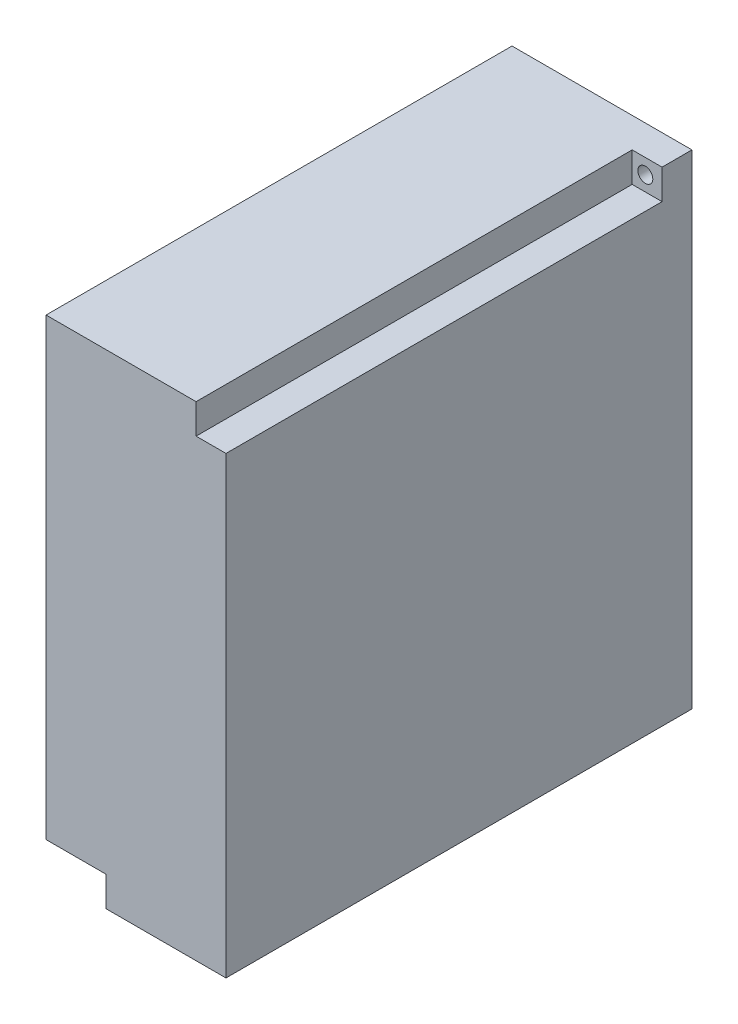
SolidWorks part; units mm, degrees
material "45#"
ref_plane "Front Plane" through (0, 0, 0) normal (0, 0, 1) x (1, 0, 0)
ref_plane "Top Plane" through (0, 0, 0) normal (0, 1, 0) x (1, 0, 0)
ref_plane "Right Plane" through (0, 0, 0) normal (1, 0, 0) x (0, 0, -1)
sketch "Sketch1" plane through (0, 0, 0) normal (0, 0, 1) x (1, 0, 0)
  line L0 (-30.1, 81) -> (30.1, -81) construction
  line L1 (-30.1, 81) -> (30.1, 81)
  line L2 (-30.1, 81) -> (-30.1, -81)
  line L3 (-30.1, -81) -> (30.1, -81)
  line L4 (30.1, 81) -> (30.1, -81)
  dimension "D1" = 60.2
  dimension "D2" = 162
extrude "Extrude1" add sketch "Sketch1" along normal blind 155.9
sketch "Sketch2" plane through (0, 0, 155.9) normal (0, 0, 1) x (1, 0, 0)
  line L1 (-30.1, -81) -> (-10.1, -81)
  line L2 (-30.1, -81) -> (-30.1, -71)
  line L3 (-30.1, -71) -> (-10.1, -71)
  line L4 (-10.1, -81) -> (-10.1, -71)
  line L5 (30.1, 81) -> (20.1, 81)
  line L6 (30.1, 81) -> (30.1, 71)
  line L7 (30.1, 71) -> (20.1, 71)
  line L8 (20.1, 81) -> (20.1, 71)
  dimension "D1" = 10
  dimension "D2" = 10
  dimension "D3" = 20
extrude "Cut-Extrude1" cut sketch "Sketch2" against normal blind 145.9
sketch "Sketch3" plane through (0, 0, 155.9) normal (0, 0, 1) x (1, 0, 0)
  line L0 (-24.5, 76) -> (24.5, -76) construction
  line L1 (-24.5, 76) -> (24.5, 76) construction
  line L2 (-24.5, 76) -> (-24.5, -76) construction
  line L3 (-24.5, -76) -> (24.5, -76) construction
  line L4 (24.5, 76) -> (24.5, -76) construction
  circle A0 centre (24.5, 76) radius 2.5
  circle A1 centre (-24.5, -76) radius 2.5
  dimension "D3" = 5
  dimension "D1" = 49
  dimension "D2" = 152
extrude "Cut-Extrude2" cut sketch "Sketch3" against normal through all
